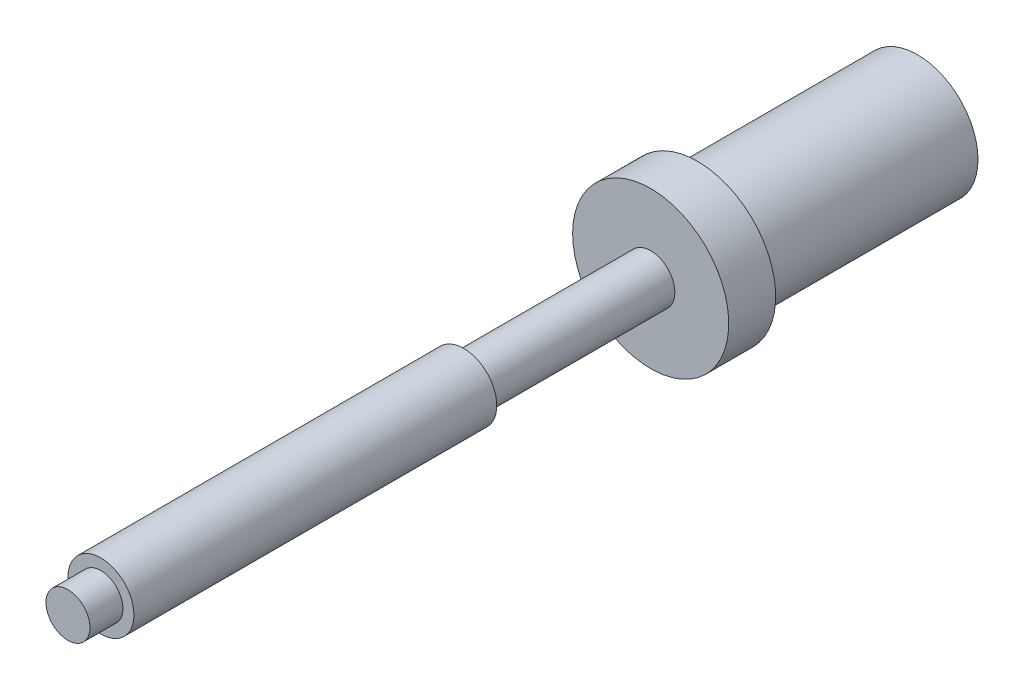
SolidWorks part; units mm, degrees
ref_plane "Front Plane" through (0, 0, 0) normal (0, 0, 1) x (1, 0, 0)
ref_plane "Top Plane" through (0, 0, 0) normal (0, 1, 0) x (1, 0, 0)
ref_plane "Right Plane" through (0, 0, 0) normal (1, 0, 0) x (0, 0, -1)
sketch "Sketch1" plane through (0, 0, 0) normal (0, 0, 1) x (1, 0, 0)
  circle A0 centre (0, 0) radius 27.5
  circle A1 centre (0, 0) radius 17.5
  dimension "D1" = 10
  dimension "D2" = 35
extrude "Boss-Extrude1" add sketch "Sketch1" along normal blind 100
sketch "Sketch2" plane through (0, 0, 100) normal (0, 0, 1) x (1, 0, 0)
  circle A0 centre (0, 0) radius 35.5
  circle A1 centre (0, 0) radius 27.5 construction
  dimension "D1" = 8
extrude "Boss-Extrude2" add sketch "Sketch2" along normal blind 21.35
sketch "Sketch3" plane through (0, 0, 121.35) normal (0, 0, 1) x (1, 0, 0)
  circle A0 centre (0, 0) radius 11
  dimension "D1" = 22
extrude "Boss-Extrude3" add sketch "Sketch3" along normal blind 85
sketch "Sketch4" plane through (0, 0, 206.35) normal (0, 0, 1) x (1, 0, 0)
  circle A0 centre (0, 0) radius 15
  dimension "D1" = 30
extrude "Boss-Extrude4" add sketch "Sketch4" along normal blind 165
sketch "Sketch5" plane through (0, 0, 371.35) normal (0, 0, 1) x (1, 0, 0)
  circle A0 centre (0, 0) radius 10
  dimension "D1" = 20
extrude "Boss-Extrude5" add sketch "Sketch5" along normal blind 15
equation "\"A\"= \"代号代码\""
equation "\"B\"= \"名称代码\""
